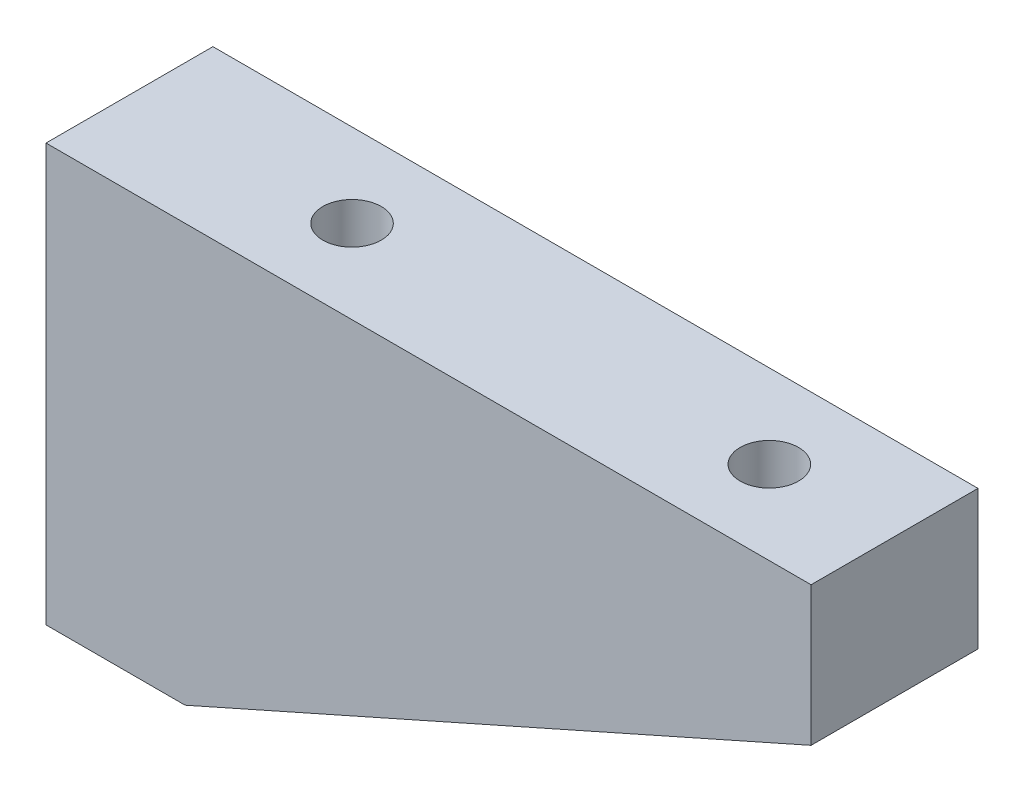
from build123d import *

# Parameters (mm, degrees)
EXTRUDE_1_DEPTH        = 12
HOLE_WIZARD_M5_1_D     = 4.2
HOLE_WIZARD_M5_1_DEPTH = 10
HOLE_WIZARD_M5_1_TIP   = 1.2618073
HOLE_WIZARD_M5_2_D     = 4.2
HOLE_WIZARD_M5_2_DEPTH = 10
HOLE_WIZARD_M5_2_TIP   = 1.2618073


with BuildPart() as part:
    # 草图1 → 凸台-拉伸1 (new body)
    with BuildSketch(Plane.XY):
        Polygon((-30.106749708, 4.118589161), (-40.106749708, 4.118589161), (-40.106749708, 34.118589161), (14.893250292, 34.118589161), (14.893250292, 24.118589161), align=None)
    extrude(amount=EXTRUDE_1_DEPTH)

    # M5 螺纹孔1
    with Locations(Plane(origin=(-24.106749708, 34.118589161, 6), x_dir=(0, 0, 1), z_dir=(0, 1, 0))):
        with Locations((0, 0), (0, 30)):
            Hole(HOLE_WIZARD_M5_1_D / 2, depth=HOLE_WIZARD_M5_1_DEPTH)
            with Locations((0, 0, -(HOLE_WIZARD_M5_1_DEPTH + HOLE_WIZARD_M5_1_TIP / 2))):  # 118° drill point
                Cone(0, HOLE_WIZARD_M5_1_D / 2, HOLE_WIZARD_M5_1_TIP, mode=Mode.SUBTRACT)

    # M5 螺纹孔2
    with Locations(Plane(origin=(-40.106749708, 9.118589161, 6), x_dir=(0, 0, -1), z_dir=(-1, 0, 0))):
        with Locations((0, 0), (0, -20)):
            Hole(HOLE_WIZARD_M5_2_D / 2, depth=HOLE_WIZARD_M5_2_DEPTH)
            with Locations((0, 0, -(HOLE_WIZARD_M5_2_DEPTH + HOLE_WIZARD_M5_2_TIP / 2))):  # 118° drill point
                Cone(0, HOLE_WIZARD_M5_2_D / 2, HOLE_WIZARD_M5_2_TIP, mode=Mode.SUBTRACT)


solid = part.part
